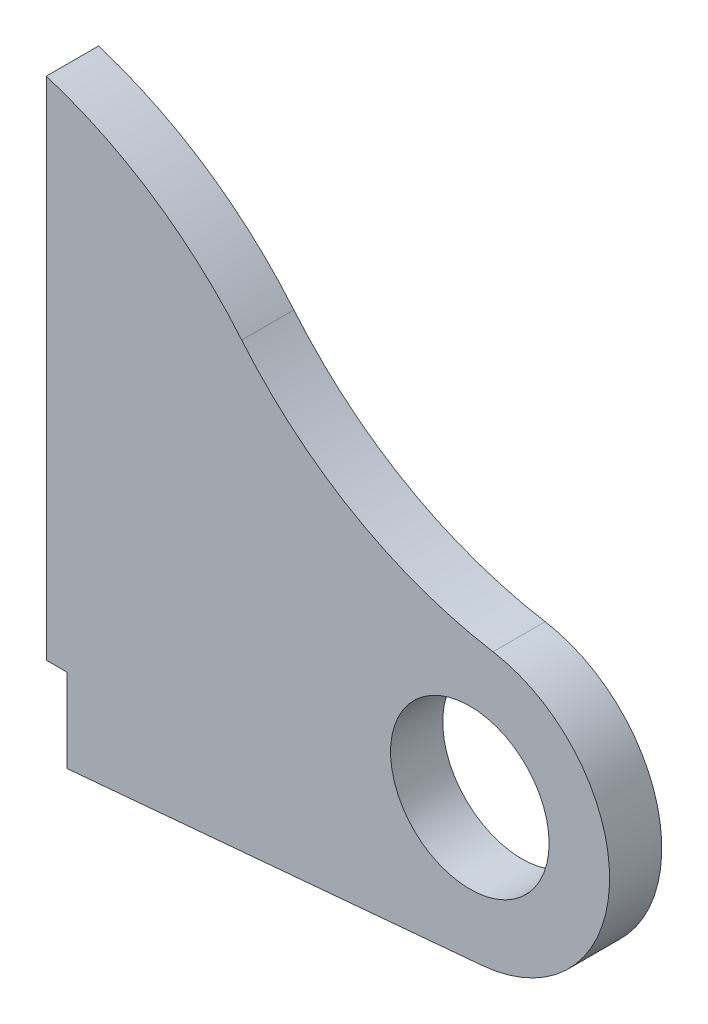
SolidWorks part; units mm, degrees
ref_plane "Front Plane" through (0, 0, 0) normal (0, 0, 1) x (1, 0, 0)
ref_plane "Top Plane" through (0, 0, 0) normal (0, 1, 0) x (1, 0, 0)
ref_plane "Right Plane" through (0, 0, 0) normal (1, 0, 0) x (0, 0, -1)
sketch "Sketch1" plane through (0, 0, 0) normal (0, 0, 1) x (1, 0, 0)
  line L0 (-203, 198) -> (-203, -44.5)
  line L1 (-203, -44.5) -> (-193, -44.5)
  line L2 (-193, -44.5) -> (-193, -84.5)
  line L3 (-193, -84.5) -> (5.9589, -66.7345)
  line L4 (-263, 44.1812) -> (-263, -29.7569) construction
  arc A0 (5.9589, -66.7345) -> (11.1099, 66.0725) centre (0, 0) ccw
  arc A1 (-109.3632, 135.2579) -> (-203, 198) centre (-263, 7.2122) ccw
  arc A2 (-109.3632, 135.2579) -> (11.1099, 66.0725) centre (44.2737, 263.3037) ccw
  circle A3 centre (0, 0) radius 38
  dimension "D1" = 134
  dimension "D8" = 400
  dimension "D9" = 400
  dimension "D10" = 76
  dimension "D2" = 198
  dimension "D3" = 203
  dimension "D4" = 242.5
  dimension "D5" = 10
  dimension "D6" = 40
  dimension "D7" = 60
extrude "Boss-Extrude1" add sketch "Sketch1" along normal blind 25
